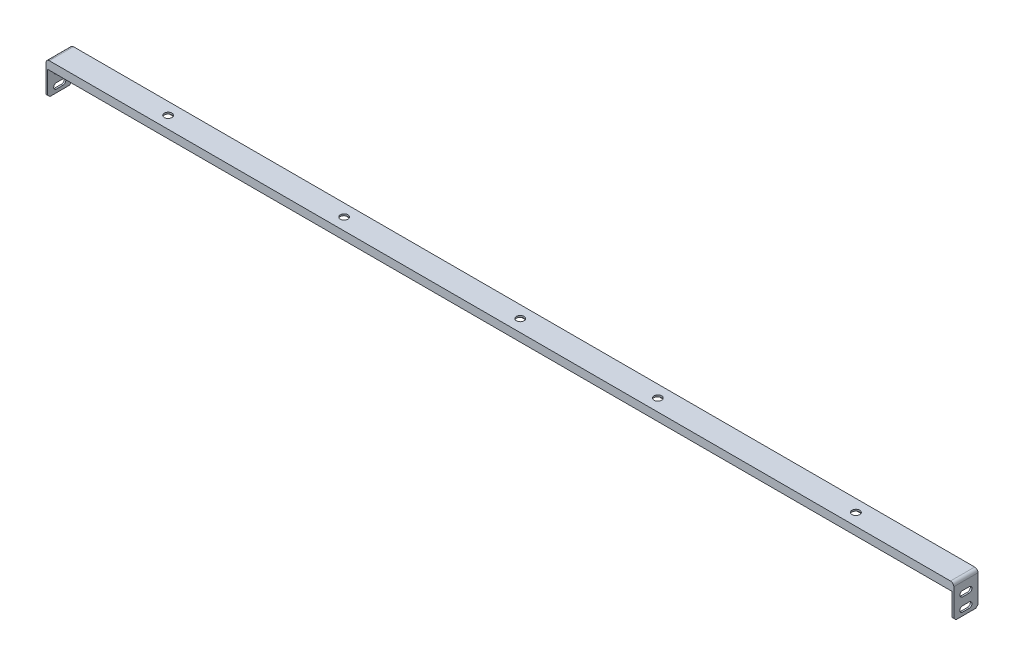
SolidWorks part; units mm, degrees
ref_plane "前视" through (0, 0, 0) normal (0, 0, 1) x (1, 0, 0)
ref_plane "上视" through (0, 0, 0) normal (0, 1, 0) x (1, 0, 0)
ref_plane "右视" through (0, 0, 0) normal (1, 0, 0) x (0, 0, -1)
sketch "草图1" plane through (0, 0, 0) normal (0, 0, 1) x (1, 0, 0)
  line L0 (0, 0) -> (0, 30)
  line L1 (0, 30) -> (825, 30)
  line L2 (825, 30) -> (825, 0)
  line L3 (825, 0) -> (823.5, 0)
  line L4 (823.5, 0) -> (823.5, 28.5)
  line L5 (823.5, 28.5) -> (1.5, 28.5)
  line L6 (1.5, 28.5) -> (1.5, 0)
  line L7 (1.5, 0) -> (0, 0)
  dimension "D1" = 1.5
  dimension "D2" = 1.5
  dimension "D3" = 825
  dimension "D4" = 30
extrude "凸台-拉伸1" add sketch "草图1" along normal blind 22
sketch "草图2" plane through (0, 0, 22) normal (0, 0, 1) x (1, 0, 0)
  line L0 (823.5, 28.5) -> (823.5, 0) construction
  line L1 (1.5, 28.5) -> (823.5, 28.5)
  line L2 (1.5, 28.5) -> (1.5, 22.5)
  line L3 (1.5, 22.5) -> (823.5, 22.5)
  line L4 (823.5, 28.5) -> (823.5, 22.5)
  dimension "D1" = 6
extrude "凸台-拉伸2" add sketch "草图2" against normal blind 2
sketch "草图3" plane through (0, 0, 0) normal (0, 0, -1) x (-1, 0, 0)
  line L1 (-823.5, 28.5) -> (-1.5, 28.5)
  line L2 (-823.5, 28.5) -> (-823.5, 22.5)
  line L3 (-823.5, 22.5) -> (-1.5, 22.5)
  line L4 (-1.5, 28.5) -> (-1.5, 22.5)
extrude "凸台-拉伸3" add sketch "草图3" against normal blind 2
sketch "草图5" plane through (0, 0, 0) normal (-1, 0, 0) x (0, 0, 1)
  line L0 (8, 17.5) -> (14, 17.5) construction
  line L1 (8, 20) -> (14, 20)
  line L2 (8, 15) -> (14, 15)
  line L3 (8, 5.5) -> (14, 5.5) construction
  line L4 (8, 8) -> (14, 8)
  line L5 (8, 3) -> (14, 3)
  line L6 (11, 0) -> (11, 10.0046) construction
  line L7 (22, 0) -> (0, 0) construction
  arc A0 (8, 20) -> (8, 15) centre (8, 17.5) ccw
  arc A1 (14, 15) -> (14, 20) centre (14, 17.5) ccw
  arc A2 (8, 8) -> (8, 3) centre (8, 5.5) ccw
  arc A3 (14, 3) -> (14, 8) centre (14, 5.5) ccw
  point P2 (11, 17.5)
  point P7 (11, 5.5)
  dimension "D1" = 5
  dimension "D2" = 5.5
  dimension "D3" = 12
  dimension "D4" = 6
extrude "切除-拉伸1" cut sketch "草图5" against normal through all
chamfer "倒角1" distance 2 angle 45 4 edges at (824.25, 0, 22) (824.25, 0, 0) (0.75, 0, 0) (0.75, 0, 22)
fillet "圆角1" radius 3 2 edges at (825, 30, 11) (0, 30, 11)
hole_wizard "Ø7.0 (7) 直径孔1" positions "草图7" profile "草图6" hole size "Ø7.0" standard "Gb" end condition through all
sketch "草图7" plane through (0, 28.5, 0) normal (0, -1, 0) x (-1, 0, 0)
  line L0 (-823.5, -11) -> (51.9242, -11) construction
  line L1 (-823.5, -20) -> (-823.5, -2) construction
  line L3 (-825, -20) -> (-825, -2) construction
  line L4 (0, -20) -> (0, -2) construction
  point P0 (-100, -11)
  point P2 (-260, -11)
  point P4 (-420, -11)
  point P6 (-545, -11)
  point P8 (-725, -11)
  dimension "D1" = 180
  dimension "D2" = 100
  dimension "D3" = 160
  dimension "D4" = 160
  dimension "D5" = 100
sketch "草图6" plane through (100, 28.5, 11) normal (1, 0, 0) x (0, 0, -1)
  line L0 (0, 0) -> (0, 1.5)
  line L1 (0, 1.5) -> (3.5, 1.5)
  line L2 (3.5, 1.5) -> (3.5, 0)
  line L5 (3.5, 0) -> (0, 0)
  line L11 (0, -6.35) -> (0, 107.95) construction
  dimension "通孔孔直径" = 7
  dimension "通孔孔深度" = 1.5
